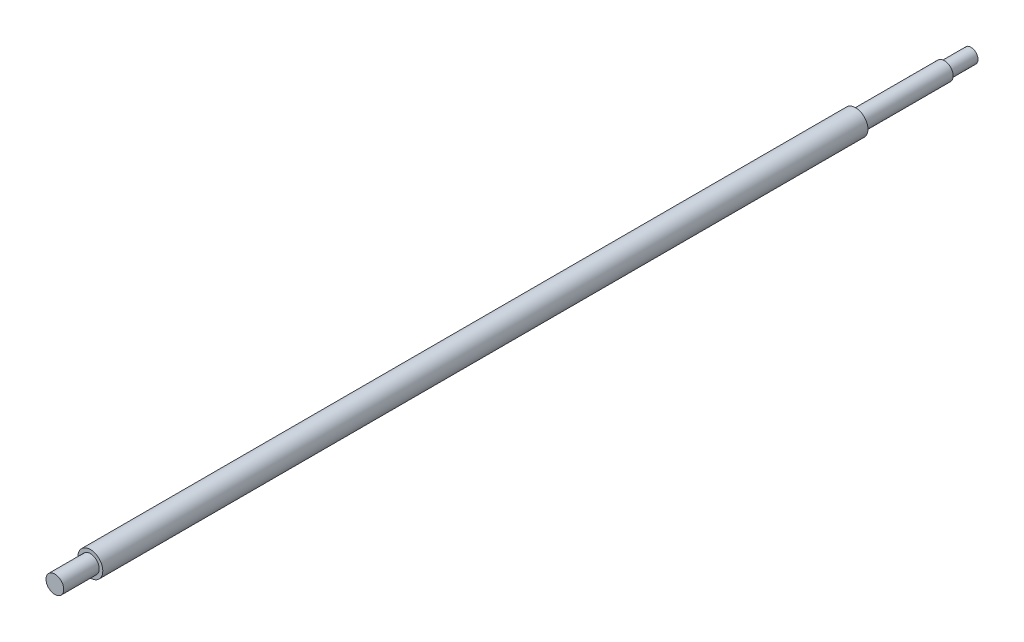
from build123d import *

# Parameters (mm, degrees)
SKETCH1_R           = 7
BOSS_EXTRUDE1_DEPTH = 431
SKETCH2_R           = 5
BOSS_EXTRUDE2_DEPTH = 20
BOSS_EXTRUDE3_START = 50
SKETCH3_R           = 5
BOSS_EXTRUDE3_DEPTH = 50
SKETCH4_R           = 4
BOSS_EXTRUDE4_DEPTH = 15


with BuildPart() as part:
    # Sketch1 → Boss-Extrude1 (new body)
    with BuildSketch(Plane.XY):
        Circle(SKETCH1_R)
    extrude(amount=BOSS_EXTRUDE1_DEPTH)

    # Sketch2 → Boss-Extrude2 (add)
    with BuildSketch(Plane.XY.offset(431)):
        Circle(SKETCH2_R)
    extrude(amount=BOSS_EXTRUDE2_DEPTH)

    # Sketch3 → Boss-Extrude3 (add)
    with BuildSketch(Plane(origin=(0, 0, 0), x_dir=(-1, 0, 0), z_dir=(0, 0, -1)).offset(BOSS_EXTRUDE3_START)):
        with Locations(Location((0, 0, 0), (0, 0, 180))):
            Circle(SKETCH3_R)
    extrude(amount=-BOSS_EXTRUDE3_DEPTH)

    # Sketch4 → Boss-Extrude4 (add)
    with BuildSketch(Plane(origin=(0, 0, -50), x_dir=(-1, 0, 0), z_dir=(0, 0, -1))):
        Circle(SKETCH4_R)
    extrude(amount=BOSS_EXTRUDE4_DEPTH)


solid = part.part
